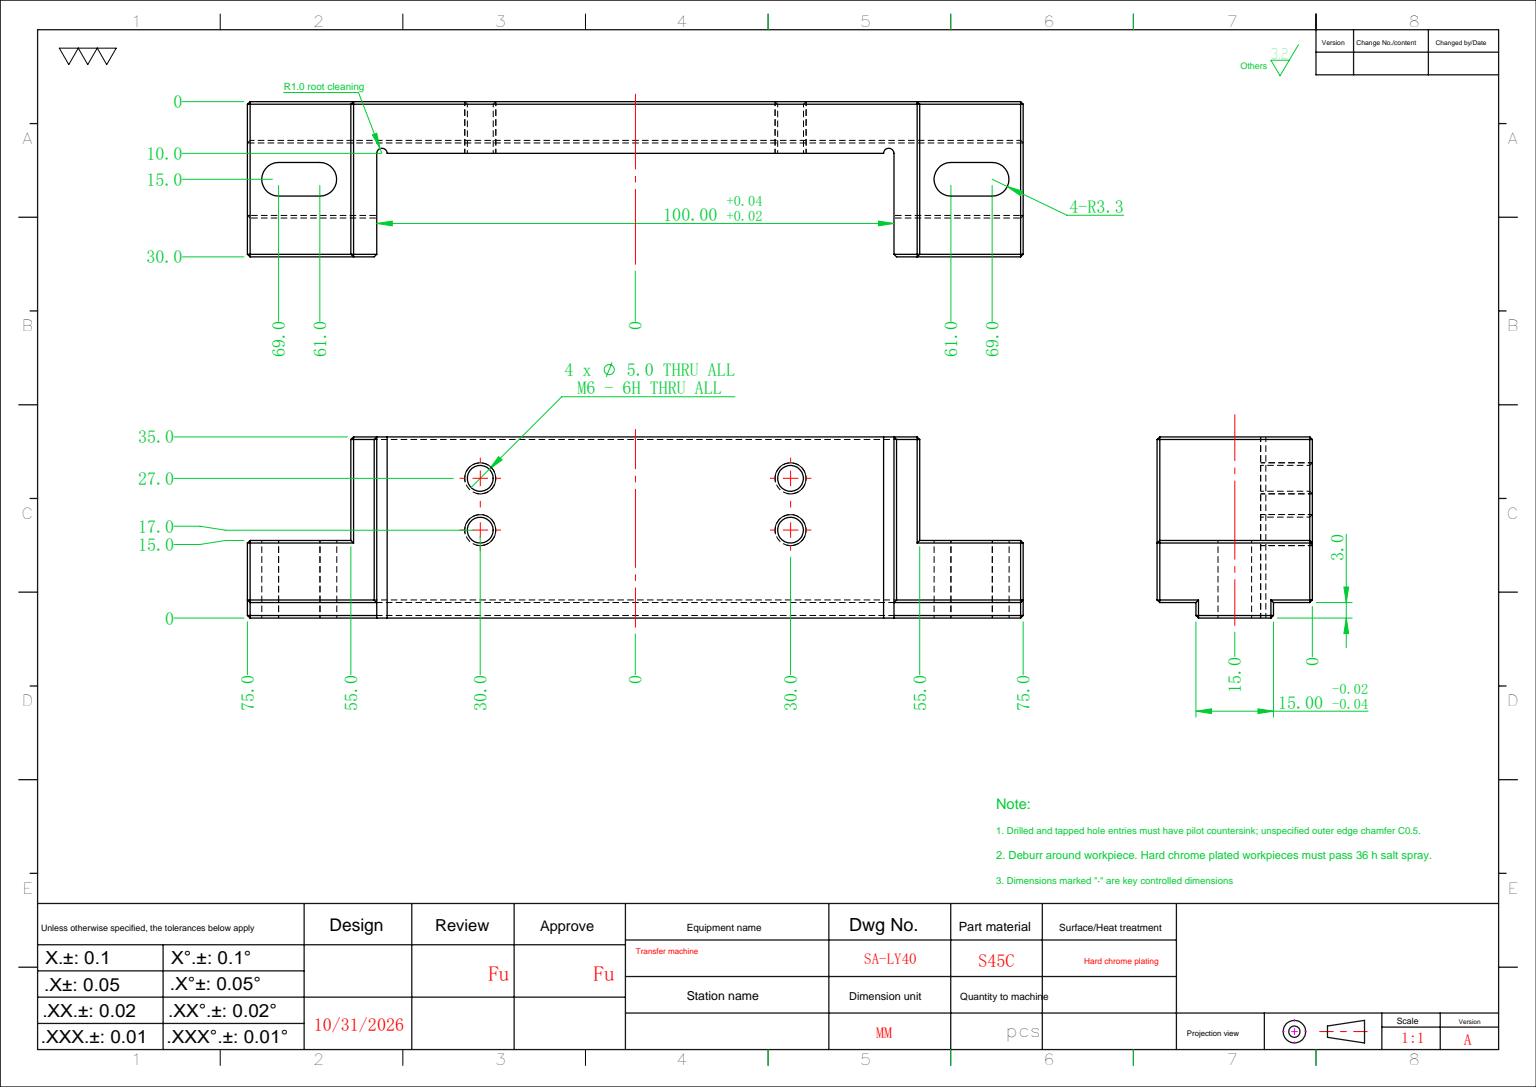
from build123d import *

# Parameters (mm, degrees)
EXTRUDE_1_DEPTH        = 15
SKETCH_2_W             = 7.5
SKETCH_2_H             = 3
CUT_EXTRUDE_1_DEPTH    = 155.757875405
SKETCH_3_W             = 100
SKETCH_3_H             = 20
CUT_EXTRUDE_2_DEPTH    = 85.113019206
CUT_EXTRUDE_3_DEPTH    = 30
HOLE_WIZARD_M6_1_D     = 5
PATTERN_LINEAR_1_COUNT = 2
PATTERN_LINEAR_1_PITCH = 10
CHAMFER_1_SIZE         = 0.5
SKETCH_7_R             = 1
CUT_EXTRUDE_4_DEPTH    = 85.113019206


with BuildPart() as part:
    # 草图1 → 凸台-拉伸1 (new, symmetric)
    with BuildSketch(Plane.XY):
        Polygon((-75, 0), (-75, 15), (-55, 15), (-55, 35), (55, 35), (55, 15), (75, 15), (75, 0), align=None)
    extrude(amount=EXTRUDE_1_DEPTH, both=True)

    # 草图2 → 切除-拉伸1 (cut, through all)
    with BuildSketch(Plane.ZY.offset(75)):
        with Locations((-11.25, 1.5)):
            Rectangle(SKETCH_2_W, SKETCH_2_H)
        with Locations((11.25, 1.5)):
            Rectangle(SKETCH_2_W, SKETCH_2_H)
    extrude(amount=-CUT_EXTRUDE_1_DEPTH, mode=Mode.SUBTRACT)

    # 草图3 → 切除-拉伸2 (cut, through all)
    with BuildSketch(Plane(origin=(0, 35, 0), x_dir=(1, 0, 0), z_dir=(0, 1, 0))):
        with Locations((0, -5)):
            Rectangle(SKETCH_3_W, SKETCH_3_H)
    extrude(amount=-CUT_EXTRUDE_2_DEPTH, mode=Mode.SUBTRACT)

    # 草图4 → 切除-拉伸3 (cut)
    with BuildSketch(Plane(origin=(0, 15, 0), x_dir=(1, 0, 0), z_dir=(0, 1, 0))):
        with BuildLine():
            Line((61, 3.25), (69, 3.25))
            ThreePointArc((69, 3.25), (72.25, 0), (69, -3.25))
            Line((69, -3.25), (61, -3.25))
            ThreePointArc((61, -3.25), (57.75, 0), (61, 3.25))
        make_face()
        with BuildLine():
            Line((-61, 3.25), (-69, 3.25))
            ThreePointArc((-69, 3.25), (-72.25, 0), (-69, -3.25))
            Line((-69, -3.25), (-61, -3.25))
            ThreePointArc((-61, -3.25), (-57.75, 0), (-61, 3.25))
        make_face()
    extrude(amount=-CUT_EXTRUDE_3_DEPTH, mode=Mode.SUBTRACT)

    # M6 螺纹孔1 (through all)
    with Locations(Plane.XY.offset(-5)):
        with Locations((-30, 17), (30, 17)):
            hole_wizard_m6_1 = Hole(HOLE_WIZARD_M6_1_D / 2)

    # 阵列(线性)1: M6 螺纹孔1 ×2
    with Locations(*[(0, i * PATTERN_LINEAR_1_PITCH, 0) for i in range(1, PATTERN_LINEAR_1_COUNT)]):
        add(hole_wizard_m6_1, mode=Mode.SUBTRACT)

    # 倒角1
    chamfer_1_edges = [part.edges().sort_by_distance(p)[0] for p in [
        (55, 25, -15),
        (65, 15, -15),
        (32.5, 17, -15),
        (-27.5, 17, -15),
        (32.5, 27, -15),
        (65, 15, 15),
        (-27.5, 27, -15),
        (-75, 15, 0),
        (-55, 35, 0),
        (55, 35, 0),
        (75, 15, 0),
        (55, 25, 15),
        (52.5, 35, 15),
        (75, 9, -15),
        (-55, 25, 15),
        (75, 9, 15),
        (-75, 0, 0),
        (-65, 15, 15),
        (75, 0, 0),
        (75, 3, -11.25),
        (-75, 9, 15),
        (0, 3, -15),
        (75, 1.5, -7.5),
        (0, 0, -7.5),
        (-75, 1.5, -7.5),
        (-75, 3, -11.25),
        (75, 1.5, 7.5),
        (62.5, 0, 7.5),
        (75, 3, 11.25),
        (62.5, 3, 15),
        (-75, 3, 11.25),
        (-75, 1.5, 7.5),
        (-62.5, 3, 15),
        (-62.5, 0, 7.5),
        (-52.5, 35, 15),
        (-50, 19, 15),
        (50, 19, 15),
        (-75, 9, -15),
        (-65, 15, -15),
        (-55, 25, -15),
        (0, 35, -15),
    ]]
    chamfer(chamfer_1_edges, length=CHAMFER_1_SIZE)

    # 草图7 → 切除-拉伸4 (cut, through all)
    with BuildSketch(Plane(origin=(0, 35, 0), x_dir=(1, 0, 0), z_dir=(0, 1, 0))):
        with Locations((-49, 5)):
            Circle(SKETCH_7_R)
        with Locations((49, 5)):
            Circle(SKETCH_7_R)
    extrude(amount=-CUT_EXTRUDE_4_DEPTH, mode=Mode.SUBTRACT)


solid = part.part
